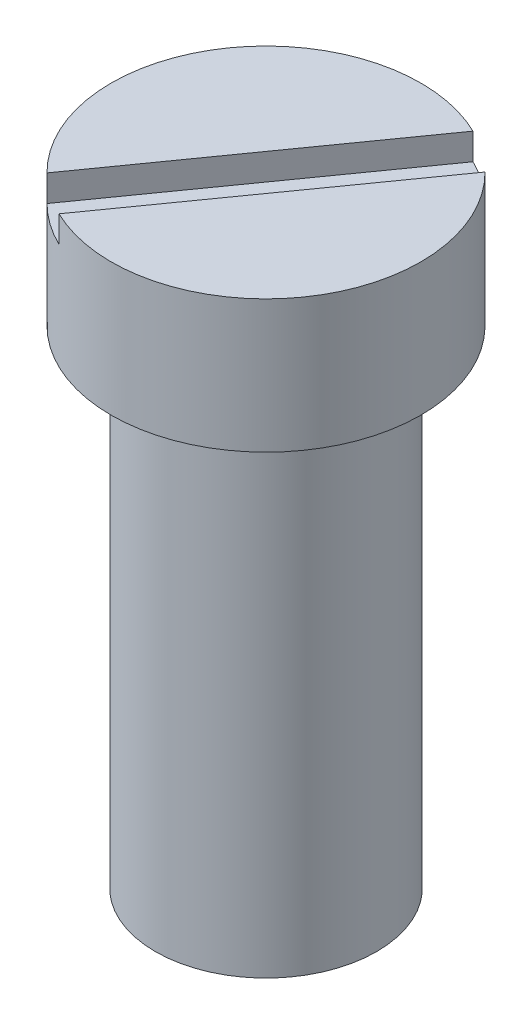
from build123d import *

# Parameters (mm, degrees)
SKETCH1_R           = 1.25
BOSS_EXTRUDE1_DEPTH = 5.5
SKETCH2_R           = 1.75
BOSS_EXTRUDE2_DEPTH = 1.5
CUT_EXTRUDE1_DEPTH  = 0.3


with BuildPart() as part:
    # Sketch1 → Boss-Extrude1 (new body)
    with BuildSketch(Plane(origin=(0, 0, 0), x_dir=(1, 0, 0), z_dir=(0, 1, 0))):
        with Locations(Location((0, 0, 0), (0, 0, 270))):
            Circle(SKETCH1_R)
    extrude(amount=BOSS_EXTRUDE1_DEPTH)

    # Sketch2 → Boss-Extrude2 (add)
    with BuildSketch(Plane(origin=(0, 5.5, 0), x_dir=(1, 0, 0), z_dir=(0, 1, 0))):
        with Locations(Location((0, 0, 0), (0, 0, 270))):
            Circle(SKETCH2_R)
    extrude(amount=BOSS_EXTRUDE2_DEPTH)

    # Sketch3 → Cut-Extrude1 (cut)
    with BuildSketch(Plane(origin=(0, 7, 0), x_dir=(1, 0, 0), z_dir=(0, 1, 0))):
        Polygon((-1.611781927, -1.775402925), (1.143517474, 2.10766798), (1.611781927, 1.775402925), (-1.143517474, -2.10766798), align=None)
    extrude(amount=-CUT_EXTRUDE1_DEPTH, mode=Mode.SUBTRACT)


solid = part.part
